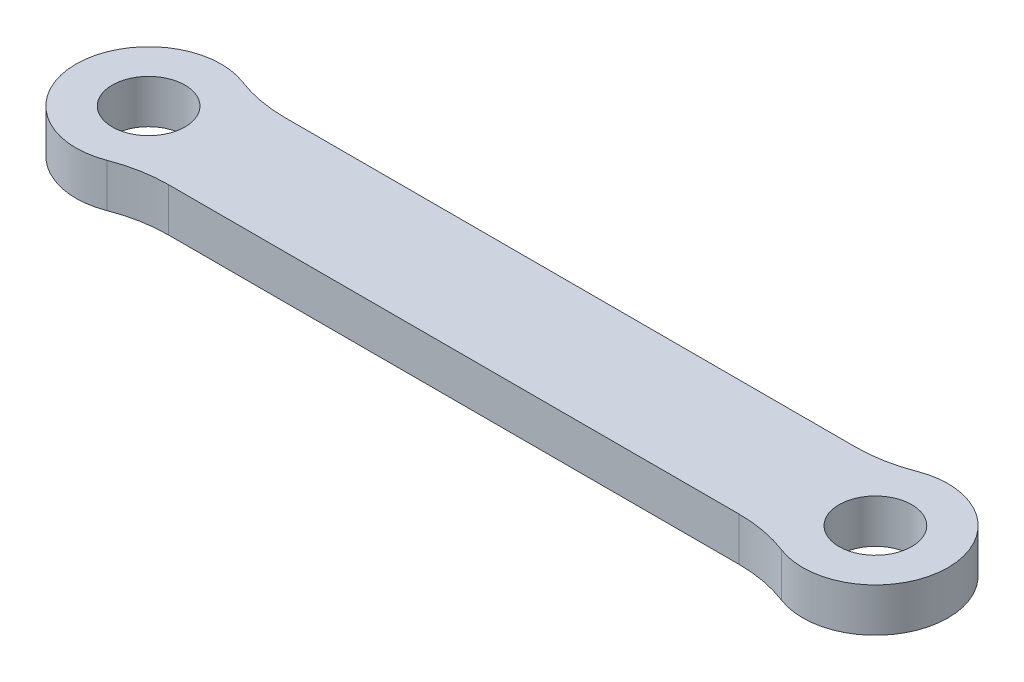
from build123d import *

# Parameters (mm, degrees)
SKETCH_1_R      = 2.5
EXTRUDE_1_DEPTH = 3
FILLET_1_R      = 10


with BuildPart() as part:
    # 草图1 → 凸台-拉伸1 (new body)
    with BuildSketch(Plane(origin=(0, 0, 0), x_dir=(1, 0, 0), z_dir=(0, 1, 0))):
        with BuildLine():
            Line((3, -4), (47, -4))
            ThreePointArc((47, -4), (55, 0), (47, 4))
            Line((47, 4), (3, 4))
            ThreePointArc((3, 4), (-5, 0), (3, -4))
        make_face()
        with Locations(Location((0, 0, 0), (0, 0, 270))):
            Circle(SKETCH_1_R, mode=Mode.SUBTRACT)
        with Locations(Location((50, 0, 0), (0, 0, 270))):
            Circle(SKETCH_1_R, mode=Mode.SUBTRACT)
    extrude(amount=EXTRUDE_1_DEPTH)

    # 圆角1
    fillet_1_edges = [part.edges().sort_by_distance(p)[0] for p in [
        (3, 1.5, -4),
        (47, 1.5, -4),
        (47, 1.5, 4),
        (3, 1.5, 4),
    ]]
    fillet(fillet_1_edges, radius=FILLET_1_R)


solid = part.part
